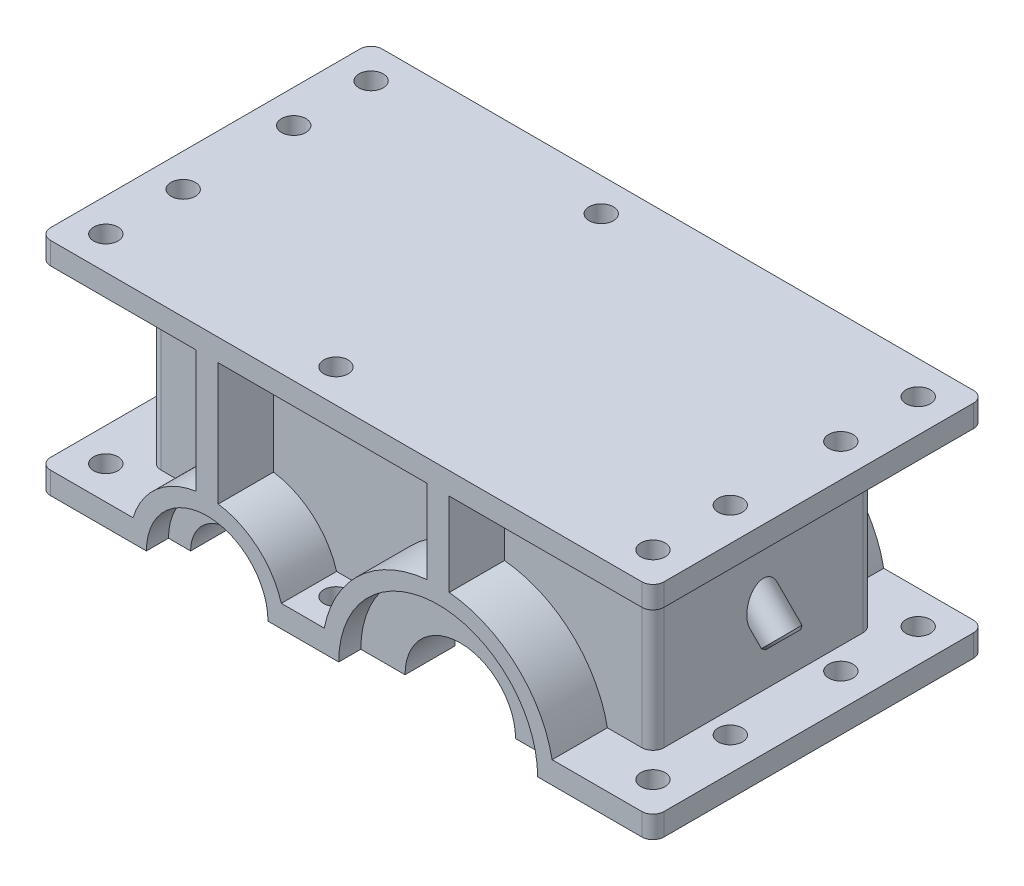
from build123d import *

# Parameters (mm, degrees)
SKETCH1_W           = 455
SKETCH1_H           = 200
BOSS_EXTRUDE1_DEPTH = 100
SHELL1_T            = -15
BOSS_EXTRUDE2_DEPTH = 20
BOSS_EXTRUDE3_DEPTH = 50
SKETCH4_R           = 90
SKETCH4_R_2         = 55
CUT_EXTRUDE1_DEPTH  = 20
SKETCH5_R           = 35
SKETCH5_R_2         = 50
CUT_EXTRUDE3_DEPTH  = 460.809743263
FILLET1_R           = 10
SKETCH6_R           = 11
CUT_EXTRUDE4_DEPTH  = 30
SKETCH7_R           = 11
BOSS_EXTRUDE4_DEPTH = 20
BOSS_EXTRUDE5_DEPTH = 10
SKETCH9_W           = 55.431100879
SKETCH9_H           = 127.178864335
BOSS_EXTRUDE6_DEPTH = 10
SKETCH11_R          = 9
CUT_EXTRUDE5_DEPTH  = 70
SKETCH12_W          = 79.277233939
SKETCH12_H          = 170
CUT_EXTRUDE6_DEPTH  = 130
CHAMFER1_SIZE       = 2


with BuildPart() as part:
    # Sketch1 → Boss-Extrude1 (new, symmetric)
    with BuildSketch(Plane.XY):
        with Locations((27.5, 100)):
            Rectangle(SKETCH1_W, SKETCH1_H)
    extrude(amount=BOSS_EXTRUDE1_DEPTH, both=True)

    # Shell1
    shell1_openings = [part.faces().sort_by_distance(p)[0] for p in [
        (27.5, 0, 0),
    ]]
    offset(amount=SHELL1_T, openings=shell1_openings, kind=Kind.INTERSECTION)

    # Sketch2 → Boss-Extrude2 (add)
    with BuildSketch(Plane(origin=(0, 0, 0), x_dir=(1, 0, 0), z_dir=(0, 1, 0))):
        Polygon((-114.985807422, 150), (-250, 150), (-250, -150), (-114.985807422, -150), (54.335521535, -150), (305, -150), (305, 150), (54.335521535, 150), align=None)
        Polygon((-114.985807422, 100), (-200, 100), (-200, -100), (-114.985807422, -100), (54.335521535, -100), (255, -100), (255, 100), (54.335521535, 100), align=None, mode=Mode.SUBTRACT)
    extrude(amount=BOSS_EXTRUDE2_DEPTH)

    # Sketch3 → Boss-Extrude3 (add)
    with BuildSketch(Plane.XY.offset(100)):
        with BuildLine():
            ThreePointArc((213.800406701, 20), (110.722766061, 105), (7.645125421, 20))
            Line((7.645125421, 20), (213.800406701, 20))
        make_face()
        with BuildLine():
            ThreePointArc((-31.196275144, 20), (-98.278314469, 70), (-165.360353794, 20))
            Line((-165.360353794, 20), (-31.196275144, 20))
        make_face()
    boss_extrude3 = extrude(amount=BOSS_EXTRUDE3_DEPTH)

    # Sketch4 → Cut-Extrude1 (cut)
    with BuildSketch(Plane.XY.offset(150)):
        with Locations((110.722766061, 0)):
            Circle(SKETCH4_R)
        with Locations((-98.278314469, 0)):
            Circle(SKETCH4_R_2)
    cut_extrude1 = extrude(amount=-CUT_EXTRUDE1_DEPTH, mode=Mode.SUBTRACT)

    # Mirror1: Boss-Extrude3, Cut-Extrude1 across plane
    add(boss_extrude3.mirror(Plane.XY))
    add(cut_extrude1.mirror(Plane.XY), mode=Mode.SUBTRACT)

    # Sketch5 → Cut-Extrude3 (cut, through all)
    with BuildSketch(Plane.XY.offset(130)):
        with Locations((-98.278314469, 0)):
            Circle(SKETCH5_R)
        with Locations((110.722766061, 0)):
            Circle(SKETCH5_R_2)
    extrude(amount=-CUT_EXTRUDE3_DEPTH, mode=Mode.SUBTRACT)

    # Fillet1
    fillet1_edges = [part.edges().sort_by_distance(p)[0] for p in [
        (-200, 110, 100),
        (255, 110, -100),
        (255, 110, 100),
        (-250, 10, -150),
        (-250, 10, 150),
        (305, 10, 150),
        (305, 10, -150),
        (-200, 110, -100),
    ]]
    fillet(fillet1_edges, radius=FILLET1_R)

    # Sketch6 → Cut-Extrude4 (cut)
    with BuildSketch(Plane(origin=(0, 20, 0), x_dir=(1, 0, 0), z_dir=(0, 1, 0))):
        with Locations(Location((-220, 120, 0), (0, 0, 270))):
            Circle(SKETCH6_R)
        with Locations(Location((-220, 50, 0), (0, 0, 270))):
            Circle(SKETCH6_R)
        with Locations(Location((-220, -50, 0), (0, 0, 270))):
            Circle(SKETCH6_R)
        with Locations(Location((-220, -120, 0), (0, 0, 270))):
            Circle(SKETCH6_R)
        with Locations(Location((275, -120, 0), (0, 0, 270))):
            Circle(SKETCH6_R)
        with Locations(Location((275, -50, 0), (0, 0, 270))):
            Circle(SKETCH6_R)
        with Locations(Location((275, 50, 0), (0, 0, 270))):
            Circle(SKETCH6_R)
        with Locations(Location((275, 120, 0), (0, 0, 270))):
            Circle(SKETCH6_R)
        with Locations(Location((-11.775574862, 120, 0), (0, 0, 270))):
            Circle(SKETCH6_R)
        with Locations(Location((-11.775574862, -120, 0), (0, 0, 270))):
            Circle(SKETCH6_R)
    extrude(amount=-CUT_EXTRUDE4_DEPTH, mode=Mode.SUBTRACT)

    # Sketch7 → Boss-Extrude4 (add)
    with BuildSketch(Plane(origin=(0, 200, 0), x_dir=(1, 0, 0), z_dir=(0, 1, 0))):
        with BuildLine():
            Line((-165.360353794, 150), (-240, 150))
            ThreePointArc((-240, 150), (-247.071067812, 147.071067812), (-250, 140))
            Line((-250, 140), (-250, -140))
            ThreePointArc((-250, -140), (-247.071067812, -147.071067812), (-240, -150))
            Line((-240, -150), (-165.360353794, -150))
            Line((-165.360353794, -150), (-31.196275144, -150))
            Line((-31.196275144, -150), (7.645125421, -150))
            Line((7.645125421, -150), (213.800406701, -150))
            Line((213.800406701, -150), (295, -150))
            ThreePointArc((295, -150), (302.071067812, -147.071067812), (305, -140))
            Line((305, -140), (305, 140))
            ThreePointArc((305, 140), (302.071067812, 147.071067812), (295, 150))
            Line((295, 150), (213.800406701, 150))
            Line((213.800406701, 150), (7.645125421, 150))
            Line((7.645125421, 150), (-31.196275144, 150))
            Line((-31.196275144, 150), (-165.360353794, 150))
        make_face()
        with Locations(Location((-220, 120, 0), (0, 0, 270))):
            Circle(SKETCH7_R, mode=Mode.SUBTRACT)
        with Locations(Location((-220, 50, 0), (0, 0, 270))):
            Circle(SKETCH7_R, mode=Mode.SUBTRACT)
        with Locations(Location((-220, -50, 0), (0, 0, 270))):
            Circle(SKETCH7_R, mode=Mode.SUBTRACT)
        with Locations(Location((-220, -120, 0), (0, 0, 270))):
            Circle(SKETCH7_R, mode=Mode.SUBTRACT)
        with Locations(Location((-11.775574862, -120, 0), (0, 0, 270))):
            Circle(SKETCH7_R, mode=Mode.SUBTRACT)
        with Locations(Location((-11.775574862, 120, 0), (0, 0, 270))):
            Circle(SKETCH7_R, mode=Mode.SUBTRACT)
        with Locations(Location((275, 120, 0), (0, 0, 270))):
            Circle(SKETCH7_R, mode=Mode.SUBTRACT)
        with Locations(Location((275, 50, 0), (0, 0, 270))):
            Circle(SKETCH7_R, mode=Mode.SUBTRACT)
        with Locations(Location((275, -50, 0), (0, 0, 270))):
            Circle(SKETCH7_R, mode=Mode.SUBTRACT)
        with Locations(Location((275, -120, 0), (0, 0, 270))):
            Circle(SKETCH7_R, mode=Mode.SUBTRACT)
        with BuildLine():
            Line((245, 100), (-190, 100))
            ThreePointArc((-190, 100), (-197.071067812, 97.071067812), (-200, 90))
            Line((-200, 90), (-200, -90))
            ThreePointArc((-200, -90), (-197.071067812, -97.071067812), (-190, -100))
            Line((-190, -100), (245, -100))
            ThreePointArc((245, -100), (252.071067812, -97.071067812), (255, -90))
            Line((255, -90), (255, 90))
            ThreePointArc((255, 90), (252.071067812, 97.071067812), (245, 100))
        make_face(mode=Mode.SUBTRACT)
    extrude(amount=-BOSS_EXTRUDE4_DEPTH)

    # Sketch8 → Boss-Extrude5 (add, symmetric)
    with BuildSketch(Plane(origin=(110.72, 0, 0), x_dir=(0, 0, -1), z_dir=(1, 0, 0))):
        Polygon((100, 100), (150, 100), (150, 184.754608039), (95.891627804, 184.754608039), align=None)
        Polygon((-95.891627804, 184.754608039), (-100, 100), (-150, 100), (-150, 184.754608039), align=None)
    extrude(amount=BOSS_EXTRUDE5_DEPTH, both=True)

    # Sketch9 → Boss-Extrude6 (add, symmetric)
    with BuildSketch(Plane(origin=(-98.28, 0, 0), x_dir=(0, 0, -1), z_dir=(1, 0, 0))):
        with Locations((122.284449561, 122.079617257)):
            Rectangle(SKETCH9_W, SKETCH9_H)
        with Locations((-122.284449561, 122.079617257)):
            Rectangle(SKETCH9_W, SKETCH9_H)
    extrude(amount=BOSS_EXTRUDE6_DEPTH, both=True)

    # Sketch10 → Revolve1 (revolve)
    with BuildSketch(Plane.XY):
        Polygon((243.881987677, 118.884442333), (283.532474552, 79.233955458), (272.925872834, 68.62735374), (233.155728657, 108.397497917), align=None)
    revolve(axis=Axis((161.553226574, 180, 0), (0.7071067811865464, -0.7071067811865488, 0)))

    # Sketch11 → Cut-Extrude5 (cut)
    with BuildSketch(Plane(origin=(102.149259547, -102.149259547, 0), x_dir=(0, 0, -1), z_dir=(0.7071067811865465, -0.7071067811865487, 0))):
        with Locations(Location((0, 241.514602646, 0), (0, 0, 90))):
            Circle(SKETCH11_R)
    extrude(amount=-CUT_EXTRUDE5_DEPTH, mode=Mode.SUBTRACT)

    # Sketch12 → Cut-Extrude6 (cut)
    with BuildSketch(Plane.XZ):
        with Locations((200.361383031, 0)):
            Rectangle(SKETCH12_W, SKETCH12_H)
    extrude(amount=-CUT_EXTRUDE6_DEPTH, mode=Mode.SUBTRACT)

    # Chamfer1
    chamfer1_edges = [part.edges().sort_by_distance(p)[0] for p in [
        (262.319271116, 58.020752022, 0),
    ]]
    chamfer(chamfer1_edges, length=CHAMFER1_SIZE)


solid = part.part
